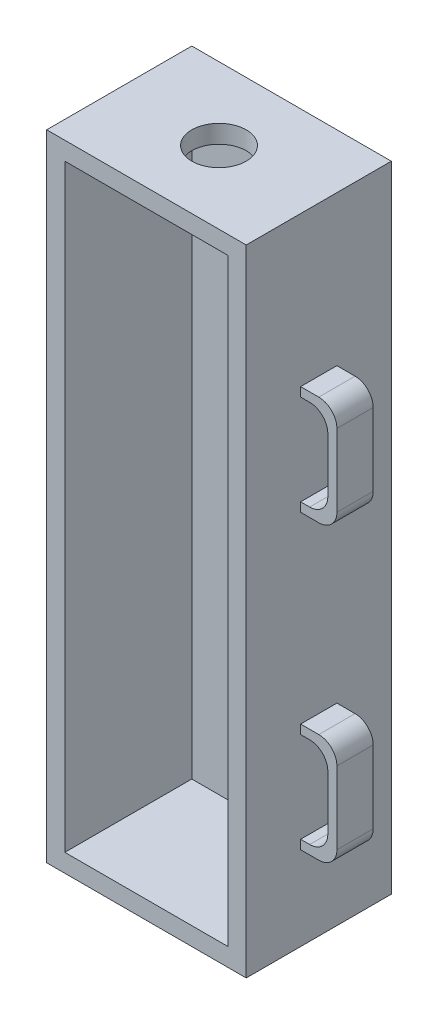
SolidWorks part; units mm, degrees
ref_plane "Front Plane" through (0, 0, 0) normal (0, 0, 1) x (1, 0, 0)
ref_plane "Top Plane" through (0, 0, 0) normal (0, 1, 0) x (1, 0, 0)
ref_plane "Right Plane" through (0, 0, 0) normal (1, 0, 0) x (0, 0, -1)
sketch "Sketch1" plane through (0, 0, 0) normal (0, 0, 1) x (1, 0, 0)
  line L3 (-174, 845) -> (-174, 495)
  line L4 (-174, 845) -> (-64, 845)
  line L6 (-64, 495) -> (-64, 845)
  line L7 (-174, 495) -> (-64, 495)
extrude "Boss-Extrude1" add sketch "Sketch1" along normal blind 80
shell "Shell1" thickness 10
sketch "Sketch2" plane through (-174, 0, 0) normal (-1, 0, 0) x (0, 0, 1)
  line L0 (40, 845) -> (40, 495) construction
  line L1 (80, 845) -> (0, 845) construction
  line L2 (80, 495) -> (0, 495) construction
  line L4 (50, 762.3635) -> (30, 762.3635)
  line L5 (50, 762.3635) -> (50, 702.3635)
  line L6 (50, 702.3635) -> (30, 702.3635)
  line L7 (30, 762.3635) -> (30, 702.3635)
  line L8 (50, 762.3635) -> (30, 702.3635) construction
  line L9 (50, 702.3635) -> (30, 762.3635) construction
  line L10 (50, 601.242) -> (30, 601.242)
  line L11 (50, 601.242) -> (50, 541.242)
  line L12 (50, 541.242) -> (30, 541.242)
  line L13 (30, 601.242) -> (30, 541.242)
  line L14 (50, 601.242) -> (30, 541.242) construction
  line L15 (50, 541.242) -> (30, 601.242) construction
  point P6 (40, 732.3635)
  point P11 (40, 571.242)
  dimension "D1" = 60
  dimension "D2" = 20
  dimension "D3" = 60
  dimension "D4" = 20
extrude "Boss-Extrude2" add sketch "Sketch2" along normal blind 20
sketch "Sketch3" plane through (0, 0, 50) normal (0, 0, 1) x (1, 0, 0)
  line L4 (-179, 596.242) -> (-174, 596.242)
  line L5 (-174, 845) -> (-174, 495) construction
  line L6 (-174, 596.242) -> (-174, 546.242)
  line L7 (-174, 546.242) -> (-179, 546.242)
  line L8 (-179, 546.242) -> (-179, 596.242)
  line L9 (-179, 596.242) -> (-189, 596.242)
  line L10 (-189, 596.242) -> (-189, 546.242)
  line L11 (-189, 546.242) -> (-179, 546.242)
  line L13 (-179, 596.242) -> (-189, 596.242)
  line L14 (-189, 596.242) -> (-189, 546.242)
  line L15 (-189, 546.242) -> (-179, 546.242)
  line L20 (-174, 757.3635) -> (-174, 707.3635)
  line L24 (-179, 707.3635) -> (-179, 757.3635)
  line L25 (-179, 757.3635) -> (-189, 757.3635)
  line L26 (-189, 757.3635) -> (-189, 707.3635)
  line L27 (-189, 707.3635) -> (-179, 707.3635)
  line L29 (-174, 757.3635) -> (-189, 757.3635)
  line L30 (-189, 757.3635) -> (-189, 707.3635)
  line L31 (-189, 707.3635) -> (-174, 707.3635)
  dimension "D2" = 5
  dimension "D1" = 5
extrude "Cut-Extrude1" cut sketch "Sketch3" against normal blind 50
fillet "Fillet1" radius 10 8 edges at (-189, 596.242, 40) (-194, 601.242, 40) (-194, 541.242, 40) (-189, 546.242, 40) (-189, 707.3635, 40) (-194, 702.3635, 40) (-189, 757.3635, 40) (-194, 762.3635, 40)
ref_plane "Plane4" through (-119, 0, 0) normal (1, 0, 0) x (0, 0, -1)
mirror "Mirror1" about plane through (-119, 0, 0) normal (1, 0, 0) of "Cut-Extrude1", "Boss-Extrude2", "Fillet1"
sketch "Sketch4" plane through (0, 845, 0) normal (0, 1, 0) x (1, 0, 0)
  line L0 (-119, -80) -> (-119, -40) construction
  line L1 (-64, -80) -> (-174, -80) construction
  line L2 (-119, -40) -> (-194, -40) construction
  line L3 (-194, -50) -> (-194, -30) construction
  circle A0 centre (-119, -40) radius 15
  dimension "D1" = 30
extrude "Cut-Extrude2" cut sketch "Sketch4" against normal blind 50
